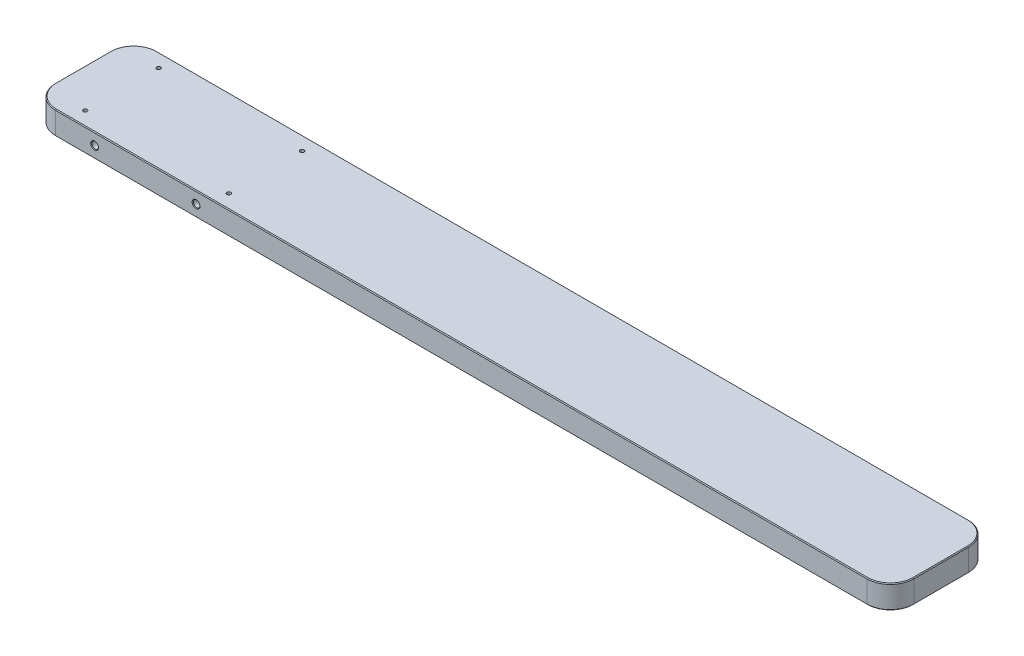
from build123d import *

# Parameters (mm, degrees)
SKETCH1_W                    = 1100
SKETCH1_H                    = 130
BOSS_EXTRUDE1_DEPTH          = 30
M6_TAPPED_HOLE1_D            = 5
M12_TAPPED_HOLE1_D           = 10.2
M12_TAPPED_HOLE1_DEPTH       = 25
M12_TAPPED_HOLE1_TIP         = 3.064389157
FILLET1_R                    = 30
CHAMFER1_SIZE                = 1
M10_TAPPED_HOLE1_D           = 8.5
M10_TAPPED_HOLE1_CSINK_D     = 10.05
M10_TAPPED_HOLE1_CSINK_ANGLE = 90


with BuildPart() as part:
    # Sketch1 → Boss-Extrude1 (new body)
    with BuildSketch(Plane(origin=(0, 0, 0), x_dir=(1, 0, 0), z_dir=(0, 1, 0))):
        Rectangle(SKETCH1_W, SKETCH1_H)
    extrude(amount=BOSS_EXTRUDE1_DEPTH)

    # M6 Tapped Hole1 (through all)
    with Locations(Plane(origin=(0, 30, 0), x_dir=(1, 0, 0), z_dir=(0, 1, 0))):
        with Locations((-316, 47), (-316, -47), (-500, 47), (-500, -47)):
            Hole(M6_TAPPED_HOLE1_D / 2)

    # M12 Tapped Hole1
    with Locations(Plane(origin=(0, 0, 0), x_dir=(-1, 0, 0), z_dir=(0, -1, 0))):
        with Locations((450, 0), (-450, 0)):
            Hole(M12_TAPPED_HOLE1_D / 2, depth=M12_TAPPED_HOLE1_DEPTH)
            with Locations((0, 0, -(M12_TAPPED_HOLE1_DEPTH + M12_TAPPED_HOLE1_TIP / 2))):  # 118° drill point
                Cone(0, M12_TAPPED_HOLE1_D / 2, M12_TAPPED_HOLE1_TIP, mode=Mode.SUBTRACT)

    # Fillet1
    fillet1_edges = [part.edges().sort_by_distance(p)[0] for p in [
        (550, 15, 65),
        (-550, 15, 65),
        (-550, 15, -65),
        (550, 15, -65),
    ]]
    fillet(fillet1_edges, radius=FILLET1_R)

    # Chamfer1
    chamfer1_edges = [part.edges().sort_by_distance(p)[0] for p in [
        (-550, 0, 0),
        (-550, 30, 0),
        (550, 0, 0),
        (0, 0, 65),
        (0, 0, -65),
        (-541.213203436, 0, 56.213203436),
        (541.213203436, 0, 56.213203436),
        (541.213203436, 0, -56.213203436),
        (-541.213203436, 0, -56.213203436),
        (0, 30, -65),
        (550, 30, 0),
        (0, 30, 65),
        (-541.213203436, 30, 56.213203436),
        (541.213203436, 30, 56.213203436),
        (541.213203436, 30, -56.213203436),
        (-541.213203436, 30, -56.213203436),
    ]]
    chamfer(chamfer1_edges, length=CHAMFER1_SIZE)

    # M10 Tapped Hole1 (through all)
    with Locations(Plane.XY.offset(65)):
        with Locations((-470, 15), (-340, 15)):
            CounterSinkHole(M10_TAPPED_HOLE1_D / 2, M10_TAPPED_HOLE1_CSINK_D / 2, counter_sink_angle=M10_TAPPED_HOLE1_CSINK_ANGLE)


solid = part.part
